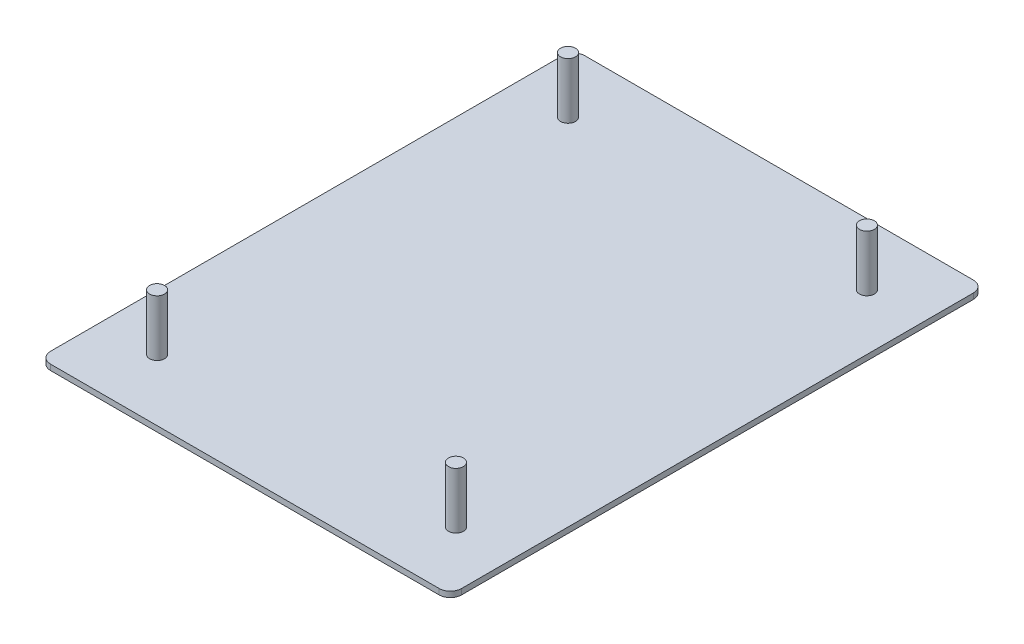
SolidWorks part; units mm, degrees
material "Q235"
ref_plane "前视基准面" through (0, 0, 0) normal (0, 0, 1) x (1, 0, 0)
ref_plane "上视基准面" through (0, 0, 0) normal (0, 1, 0) x (1, 0, 0)
ref_plane "右视基准面" through (0, 0, 0) normal (1, 0, 0) x (0, 0, -1)
sketch "草图1" plane through (0, 0, 0) normal (0, 1, 0) x (1, 0, 0)
  line L1 (0, 0) -> (110, 0)
  line L2 (0, 0) -> (0, 143)
  line L3 (0, 143) -> (110, 143)
  line L4 (110, 0) -> (110, 143)
  dimension "D1" = 110
  dimension "D2" = 143
extrude "凸台-拉伸1" add sketch "草图1" along normal blind 1.5
fillet "圆角1" radius 3 4 edges at (0, 0.75, -143) (0, 0.75, 0) (110, 0.75, -143) (110, 0.75, 0)
sketch "草图2" plane through (0, 1.5, 0) normal (0, 1, 0) x (1, 0, 0)
  line L0 (0, 140) -> (0, 3) construction
  line L3 (0, 71.5) -> (110, 71.5) construction
  line L4 (110, 3) -> (110, 140) construction
  line L5 (55, 143) -> (55, 0) construction
  line L6 (107, 143) -> (3, 143) construction
  line L7 (3, 0) -> (107, 0) construction
  circle A0 centre (15, 126.5) radius 2
  circle A1 centre (95, 16.5) radius 2
  circle A2 centre (15, 16.5) radius 2
  circle A3 centre (95, 126.5) radius 2
  dimension "D1" = 80
  dimension "D3" = 110
  dimension "D8" = 4
extrude "凸台-拉伸2" add sketch "草图2" along normal blind 15
cosmetic thread "装饰螺纹线1" parameters "D2"=3
